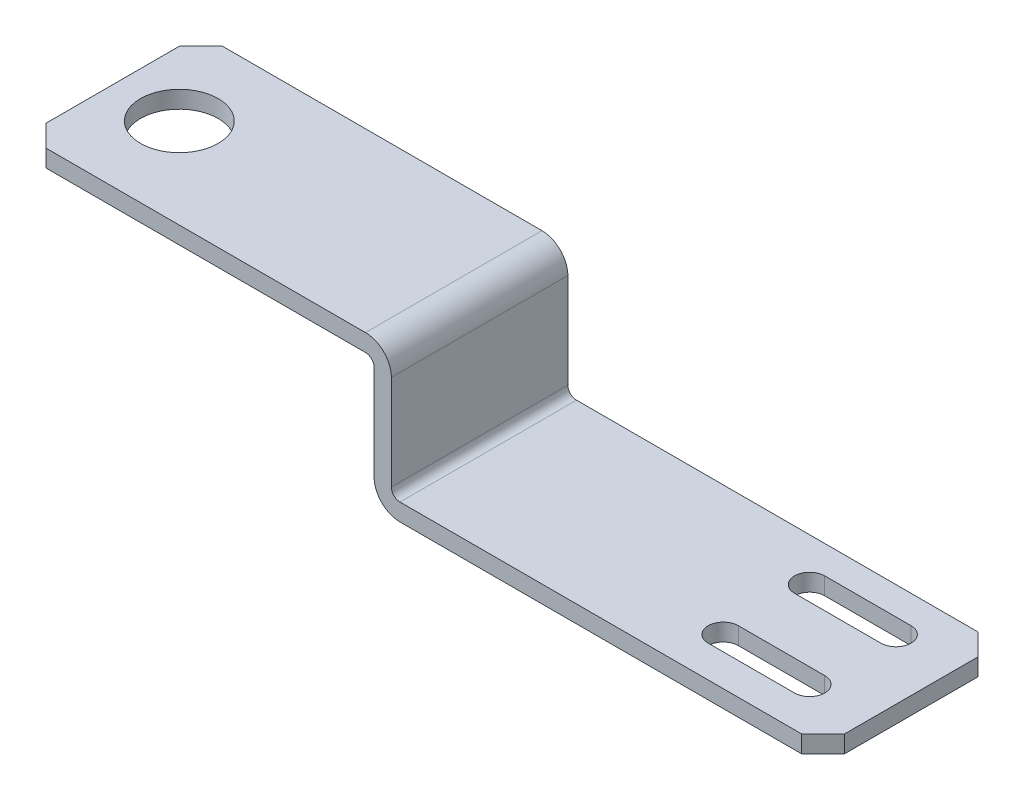
from build123d import *

# Parameters (mm, degrees)
SKETCH_1_W              = 185
SKETCH_1_H              = 40.883977901
EXTRUDE_1_DEPTH         = 34
SKETCH_2_W              = 100
SKETCH_2_H              = 30
CUT_EXTRUDE_1_DEPTH     = 192.824137295
SKETCH_3_W              = 81
SKETCH_3_H              = 30
CUT_EXTRUDE_2_DEPTH     = 192.824137295
CUT_EXTRUDE_3_DEPTH     = 193.490258582
CUT_EXTRUDE_4_DEPTH     = 192.824137295
HOLE_WIZARD_18_0_18_1_D = 18
CHAMFER_1_SIZE          = 5
FILLET_1_R              = 2
FILLET_2_R              = 6


with BuildPart() as part:
    # 草图1 → 凸台-拉伸1 (new body)
    with BuildSketch(Plane.XZ.offset(30)):
        with Locations((92.5, 20.441988951)):
            Rectangle(SKETCH_1_W, SKETCH_1_H)
    extrude(amount=-EXTRUDE_1_DEPTH)

    # 草图2 → 切除-拉伸1 (cut, through all)
    with BuildSketch(Plane(origin=(0, 0, 0), x_dir=(-1, 0, 0), z_dir=(0, 0, -1))):
        with Locations((-135, -11)):
            Rectangle(SKETCH_2_W, SKETCH_2_H)
    extrude(amount=-CUT_EXTRUDE_1_DEPTH, mode=Mode.SUBTRACT)

    # 草图3 → 切除-拉伸2 (cut, through all)
    with BuildSketch(Plane(origin=(0, 0, 0), x_dir=(-1, 0, 0), z_dir=(0, 0, -1))):
        with Locations((-40.5, -15)):
            Rectangle(SKETCH_3_W, SKETCH_3_H)
    extrude(amount=-CUT_EXTRUDE_2_DEPTH, mode=Mode.SUBTRACT)

    # 草图4 → 切除-拉伸3 (cut, through all)
    with BuildSketch(Plane.XZ.offset(30)):
        with BuildLine():
            Line((171, 13.5), (151, 13.5))
            ThreePointArc((151, 13.5), (147.5, 10), (151, 6.5))
            Line((151, 6.5), (171, 6.5))
            ThreePointArc((171, 6.5), (174.5, 10), (171, 13.5))
        make_face()
    extrude(amount=-CUT_EXTRUDE_3_DEPTH, mode=Mode.SUBTRACT)

    # 草图5 → 切除-拉伸4 (cut, through all)
    with BuildSketch(Plane(origin=(0, -26, 0), x_dir=(-1, 0, 0), z_dir=(0, 1, 0))):
        with BuildLine():
            Line((-151, 33.5), (-171, 33.5))
            ThreePointArc((-171, 33.5), (-174.5, 30), (-171, 26.5))
            Line((-171, 26.5), (-151, 26.5))
            ThreePointArc((-151, 26.5), (-147.5, 30), (-151, 33.5))
        make_face()
    extrude(amount=-CUT_EXTRUDE_4_DEPTH, mode=Mode.SUBTRACT)

    # Ø18.0 (18) 直径孔1 (through all)
    with Locations(Plane(origin=(0, 0, 0), x_dir=(-1, 0, 0), z_dir=(0, -1, 0))):
        with Locations((-15, -20)):
            Hole(HOLE_WIZARD_18_0_18_1_D / 2)

    # 倒角1
    chamfer_1_edges = [part.edges().sort_by_distance(p)[0] for p in [
        (185, -28, 0),
        (185, -28, 40.883977901),
        (0, 2, 40.883977901),
        (0, 2, 0),
    ]]
    chamfer(chamfer_1_edges, length=CHAMFER_1_SIZE)

    # 圆角1
    fillet_1_edges = [part.edges().sort_by_distance(p)[0] for p in [
        (85, -26, 20.44198895),
        (81, 0, 20.44198895),
    ]]
    fillet(fillet_1_edges, radius=FILLET_1_R)

    # 圆角2
    fillet_2_edges = [part.edges().sort_by_distance(p)[0] for p in [
        (85, 4, 20.44198895),
        (81, -30, 20.44198895),
    ]]
    fillet(fillet_2_edges, radius=FILLET_2_R)


solid = part.part
